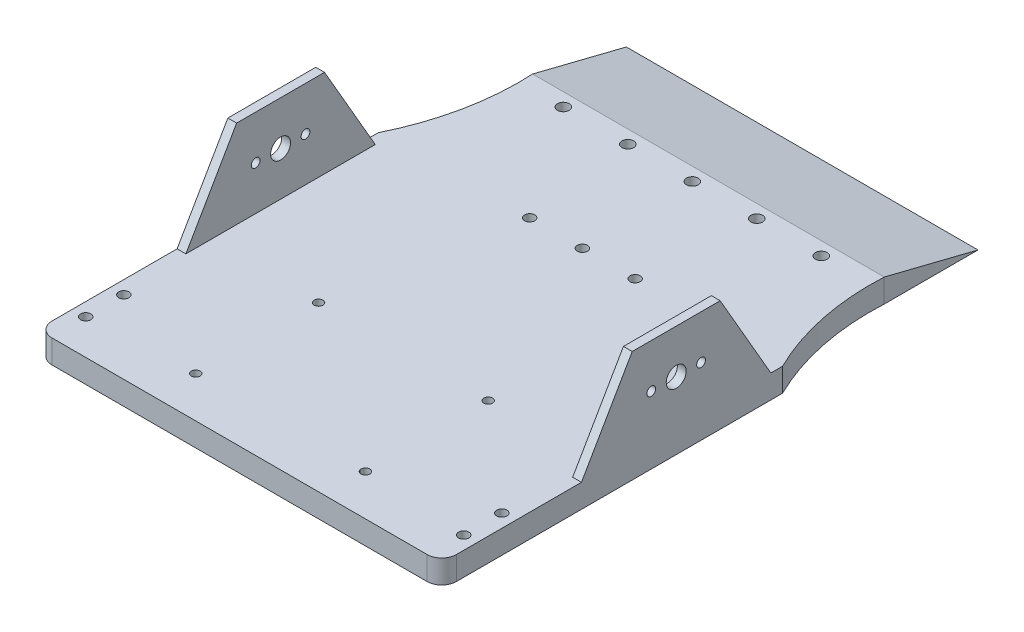
SolidWorks part; units mm, degrees
ref_plane "Front Plane" through (0, 0, 0) normal (0, 0, 1) x (1, 0, 0)
ref_plane "Top Plane" through (0, 0, 0) normal (0, 1, 0) x (1, 0, 0)
ref_plane "Right Plane" through (0, 0, 0) normal (1, 0, 0) x (0, 0, -1)
other "Configuration Table"
sketch "Sketch1" plane through (0, 0, 0) normal (0, 1, 0) x (1, 0, 0)
  line L1 (-69, -80) -> (69, -80)
  line L2 (-69, -80) -> (-69, 80)
  line L3 (-69, 80) -> (69, 80)
  line L4 (69, -80) -> (69, 80)
  line L5 (0, 80) -> (0, -80) construction
  line L6 (-69, 0) -> (69, 0) construction
  point P0 (0, 0)
  dimension "D1" = 138
  dimension "D2" = 160
extrude "Boss-Extrude1" add sketch "Sketch1" along normal blind 8
sketch "Sketch9" plane through (-69, 0, 0) normal (-1, 0, 0) x (0, 0, 1)
  line L0 (0, 0) -> (0, 60.6555) construction
  line L1 (-80, 0) -> (80, 0) construction
  line L2 (-15, 0) -> (15, 0)
  line L3 (-15, 0) -> (-15, 38)
  line L4 (-15, 38) -> (15, 38)
  line L5 (15, 0) -> (15, 38)
  line L6 (-80, 8) -> (80, 8) construction
  circle A0 centre (0, 23) radius 3.4
  circle A1 centre (0, 23) radius 8.5 construction
  circle A2 centre (8.5, 23) radius 1.5
  circle A3 centre (-8.5, 23) radius 1.5
  dimension "D3" = 6.8
  dimension "D4" = 17
  dimension "D5" = 3
  dimension "D1" = 30
  dimension "D2" = 30
  dimension "D6" = 15
extrude "Boss-Extrude4" add sketch "Sketch9" against normal blind 3
sketch "Sketch10" plane through (-69, 0, 0) normal (-1, 0, 0) x (0, 0, 1)
  line L0 (-15, 38) -> (-32.3205, 8)
  line L1 (-80, 8) -> (-15, 8) construction
  dimension "D1" = 60
rib "Rib2" sketch "Sketch10" sketch "Sketch10" thickness 3 extrusion direction parallel to sketch draft on no parameters "D1"=3
mirror "Mirror3" about plane through (0, 0, 0) normal (0, 0, 1) of "Rib2"
mirror "Mirror4" about plane through (0, 0, 0) normal (1, 0, 0) of "Mirror3", "Rib2", "Boss-Extrude4"
sketch "Sketch11" plane through (0, 8, 0) normal (0, 1, 0) x (1, 0, 0)
  line L0 (-69, -80) -> (69, -80) construction
  line L1 (-28.95, -66) -> (28.95, -66) construction
  line L2 (-28.95, -66) -> (-28.95, -24.1) construction
  line L3 (-28.95, -24.1) -> (28.95, -24.1) construction
  line L4 (28.95, -66) -> (28.95, -24.1) construction
  line L5 (0, -24.1) -> (0, -66) construction
  line L6 (-28.95, -45.05) -> (28.95, -45.05) construction
  circle A0 centre (-28.95, -24.1) radius 1.5
  circle A1 centre (28.95, -24.1) radius 1.5
  circle A2 centre (-28.95, -66) radius 1.5
  circle A3 centre (28.95, -66) radius 1.5
  point P0 (0, -45.05)
  dimension "D3" = 3
  dimension "D1" = 57.9
  dimension "D2" = 41.9
  dimension "D4" = 14
extrude "Cut-Extrude2" cut sketch "Sketch11" against normal through all both
fillet "Fillet1" radius 5 4 edges at (69, 4, -80) (-69, 4, -80) (-69, 4, 80) (69, 4, 80)
sketch "Sketch12" plane through (0, 8, 0) normal (0, 1, 0) x (1, 0, 0)
  line L0 (0, 0) -> (0, -114.3723) construction
  line L1 (-64, -80) -> (64, -80) construction
  circle A0 centre (64.5, -55) radius 1.75
  circle A1 centre (64.5, -68) radius 1.75
  dimension "D2" = 3.5
  dimension "D1" = 13
  dimension "D3" = 12
  dimension "D4" = 129
extrude "Cut-Extrude3" cut sketch "Sketch12" against normal through all both
mirror "Mirror5" about plane through (0, 0, 0) normal (1, 0, 0) of "Cut-Extrude3"
sketch "Sketch13" plane through (0, 8, 0) normal (0, 1, 0) x (1, 0, 0)
  line L0 (64, 80) -> (-64, 80) construction
  line L1 (69, 32.3205) -> (69, 75) construction
  line L2 (66, 32.3205) -> (69, 32.3205) construction
  line L3 (60, 80) -> (80.3854, 90.5857)
  line L4 (80.3854, 90.5857) -> (122.1008, 60.3291)
  line L5 (122.1008, 60.3291) -> (69, 36.3205)
  arc A0 (60, 80) -> (69, 36.3205) centre (147.8765, 75.3397) ccw
  dimension "D3" = 88
  dimension "D1" = 9
  dimension "D2" = 4
extrude "Cut-Extrude4" cut sketch "Sketch13" against normal through all both
mirror "Mirror6" about plane through (0, 0, 0) normal (1, 0, 0) of "Cut-Extrude4"
sketch "Sketch14" plane through (0, 0, 0) normal (1, 0, 0) x (0, 0, -1)
  line L0 (80, 0) -> (80, 8) construction
  line L1 (80, 0) -> (80, 8)
  line L2 (80, 8) -> (112, 0)
  line L3 (112, 0) -> (80, 0)
  line L4 (-80, 0) -> (-80, 8) construction
  dimension "D1" = 192
extrude "Boss-Extrude5" add sketch "Sketch14" along normal up to vertex (60 mm away) and the other way up to vertex (60 mm away) up to point (60, 8, -80) other way up to point (-60, 8, -80)
sketch "Sketch15" plane through (0, 0, 0) normal (0, -1, 0) x (1, 0, 0)
  line L0 (-53.5597, -75.5) -> (39.9838, -75.5) construction
  line L1 (-60, -80) -> (-60, -112) construction
  circle A0 centre (-45, -75.5) radius 2
  circle A1 centre (-23, -75.5) radius 2
  circle A2 centre (-1, -75.5) radius 2
  circle A3 centre (21, -75.5) radius 2
  circle A4 centre (43, -75.5) radius 2
  dimension "D2" = 4
  dimension "D1" = 75.5
  dimension "D3" = 15
  dimension "D4" = 5
extrude "Cut-Extrude5" cut sketch "Sketch15" against normal through all both
sketch "Sketch16" plane through (0, 8, 0) normal (0, 1, 0) x (1, 0, 0)
  line L0 (-45.7489, 37) -> (40.3558, 37) construction
  line L1 (60, 80) -> (-60, 80) construction
  line L2 (0, 0) -> (0, 37) construction
  circle A0 centre (0, 37) radius 1.75
  circle A1 centre (18, 37) radius 1.75
  circle A2 centre (-18, 37) radius 1.75
  dimension "D2" = 3.5
  dimension "D3" = 3.5
  dimension "D1" = 43
  dimension "D4" = 18
extrude "Cut-Extrude6" cut sketch "Sketch16" against normal blind 50
